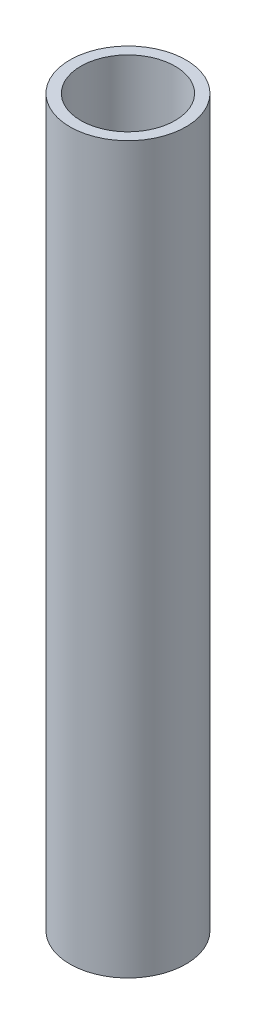
from build123d import *

# Parameters (mm, degrees)
SWEEP_THIN_PART1_PROFILE_R   = 8
SWEEP_THIN_PART1_PROFILE_R_2 = 6.5


with BuildPart() as part:
    # Sweep-Thin Part1: sweep along a path in Sketch1
    with BuildLine(Plane.XY) as sweep_thin_part1_path:
        Line((0, 0), (0, 100))
    # Sweep-Thin Part1 profile (on start of the path) → Sweep-Thin Part1 (sweep)
    with BuildSketch(Plane.ZX):
        Circle(SWEEP_THIN_PART1_PROFILE_R)
        Circle(SWEEP_THIN_PART1_PROFILE_R_2, mode=Mode.SUBTRACT)
    sweep(path=sweep_thin_part1_path.line)


solid = part.part
